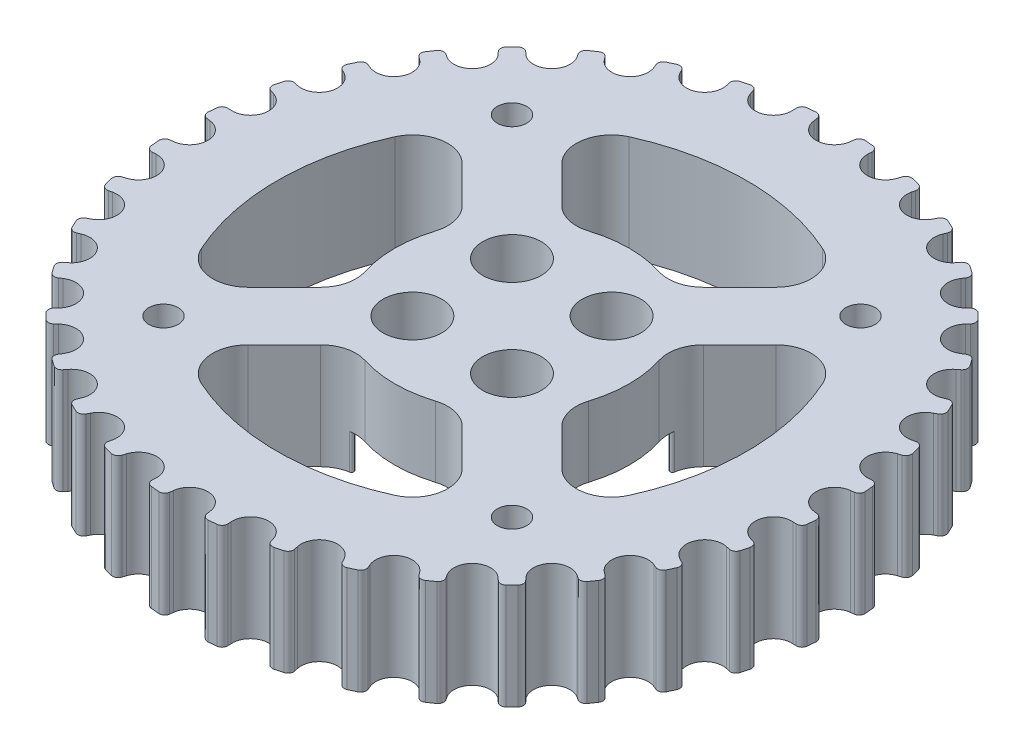
from build123d import *

# Parameters (mm, degrees)
CUT_EXTRUDE_1_DEPTH      = 46.197240435
PATTERN_CIRCULAR_1_COUNT = 36
CUT_EXTRUDE_START        = -2.5
SKETCH_3_R               = 41.846456916
CUT_EXTRUDE_2_DEPTH      = 2.5
SKETCH_4_R               = 25
EXTRUDE_1_DEPTH          = 9
CUT_EXTRUDE_START_2      = -6
SKETCH_5_R               = 29.365062609
CUT_EXTRUDE_3_DEPTH      = 6
SKETCH_6_R               = 2.5
SKETCH_6_R_2             = 1.25
CUT_EXTRUDE_4_DEPTH      = 10
SKETCH_8_R               = 10.05
CUT_EXTRUDE_6_DEPTH      = 3
FILLET_1_R               = 0.2


with BuildPart() as part:
    # 草图1 → 旋转1 (revolve)
    with BuildSketch(Plane.XY, mode=Mode.PRIVATE) as revolve_1_sk:
        Polygon((24, 0), (28.08, 0), (28.08, 9), (30.14789, 9), (30.14789, 11.5), (22.5, 11.5), (22.5, 4), (18, 4), (18, 3), (9, 3), (9, -2), (18.5, -2), (18.5, -6), (20, -6), (20, -5), (21, -5), (21, 2), (24, 2), align=None)
    revolve(revolve_1_sk.sketch.rotate(Axis((0, 0, 0), (0, 1, 0)), 90), axis=Axis((0, 0, 0), (0, 1, 0)))

    # 草图2 → 切除-拉伸1 (cut, through all)
    with BuildSketch(Plane.XZ.offset(-9)):
        with BuildLine():
            Line((-1.58417409, 27.581468475), (-1.548371997, 27.289883824))
            ThreePointArc((-1.548371997, 27.289883824), (0, 25.92), (1.548371997, 27.289883824))
            Line((1.548371997, 27.289883824), (1.58417409, 27.581468475))
            ThreePointArc((1.58417409, 27.581468475), (1.756189946, 27.894100287), (2.096432699, 28.001631559))
            ThreePointArc((2.096432699, 28.001631559), (0, 28.08), (-2.096432699, 28.001631559))
            ThreePointArc((-2.096432699, 28.001631559), (-1.756189946, 27.894100287), (-1.58417409, 27.581468475))
        make_face()
    cut_extrude_1 = extrude(amount=CUT_EXTRUDE_1_DEPTH, mode=Mode.SUBTRACT)

    # 阵列(圆周)1: 切除-拉伸1 ×36 about axis
    pattern_circular_1_axis = Axis((0, 0, 0), (0, 1, 0))
    for i in range(1, PATTERN_CIRCULAR_1_COUNT):
        add(cut_extrude_1.rotate(pattern_circular_1_axis, i * 360 / PATTERN_CIRCULAR_1_COUNT), mode=Mode.SUBTRACT)

    # 草图3 → 切除-拉伸2 (cut)
    with BuildSketch(Plane(origin=(0, 11.5, 0), x_dir=(1, 0, 0), z_dir=(0, 1, 0)).offset(CUT_EXTRUDE_START)):
        Circle(SKETCH_3_R)
    extrude(amount=CUT_EXTRUDE_2_DEPTH, mode=Mode.SUBTRACT)

    # 草图4 → 凸台-拉伸1 (add)
    with BuildSketch(Plane(origin=(0, 9, 0), x_dir=(1, 0, 0), z_dir=(0, 1, 0))):
        Circle(SKETCH_4_R)
    extrude(amount=-EXTRUDE_1_DEPTH)

    # 草图5 → 切除-拉伸3 (cut)
    with BuildSketch(Plane.XZ.offset(6).offset(CUT_EXTRUDE_START_2)):
        Circle(SKETCH_5_R)
    extrude(amount=CUT_EXTRUDE_3_DEPTH, mode=Mode.SUBTRACT)

    # 草图6 → 切除-拉伸4 (cut)
    with BuildSketch(Plane(origin=(0, 9, 0), x_dir=(1, 0, 0), z_dir=(0, 1, 0))):
        with Locations(Location((-4.242640687, 4.242640687, 0), (0, 0, 270))):
            Circle(SKETCH_6_R)
        with Locations(Location((4.242640687, 4.242640687, 0), (0, 0, 270))):
            Circle(SKETCH_6_R)
        with Locations(Location((-4.242640687, -4.242640687, 0), (0, 0, 270))):
            Circle(SKETCH_6_R)
        with Locations(Location((4.242640687, -4.242640687, 0), (0, 0, 270))):
            Circle(SKETCH_6_R)
        with Locations(Location((-14.849242405, 14.849242405, 0), (0, 0, 270))):
            Circle(SKETCH_6_R_2)
        with Locations(Location((14.849242405, 14.849242405, 0), (0, 0, 270))):
            Circle(SKETCH_6_R_2)
        with Locations(Location((14.849242405, -14.849242405, 0), (0, 0, 270))):
            Circle(SKETCH_6_R_2)
        with Locations(Location((-14.849242405, -14.849242405, 0), (0, 0, 270))):
            Circle(SKETCH_6_R_2)
        with BuildLine():
            Line((-6.033432872, 10.276073559), (-9.125901536, 13.368542223))
            ThreePointArc((-9.125901536, 13.368542223), (-9.955920686, 16.028003061), (-8.240683755, 18.223367725))
            ThreePointArc((-8.240683755, 18.223367725), (0, 20), (8.240683755, 18.223367725))
            ThreePointArc((8.240683755, 18.223367725), (9.955920686, 16.028003061), (9.125901536, 13.368542223))
            Line((9.125901536, 13.368542223), (6.033432872, 10.276073559))
            ThreePointArc((6.033432872, 10.276073559), (4.624825024, 9.483283249), (3.009317329, 9.536456848))
            ThreePointArc((3.009317329, 9.536456848), (0, 10), (-3.009317329, 9.536456848))
            ThreePointArc((-3.009317329, 9.536456848), (-4.624825024, 9.483283249), (-6.033432872, 10.276073559))
        make_face()
        with BuildLine():
            Line((-13.368542223, 9.125901536), (-10.276073559, 6.033432872))
            ThreePointArc((-10.276073559, 6.033432872), (-9.483283249, 4.624825024), (-9.536456848, 3.009317329))
            ThreePointArc((-9.536456848, 3.009317329), (-10, 0), (-9.536456848, -3.009317329))
            ThreePointArc((-9.536456848, -3.009317329), (-9.483283249, -4.624825024), (-10.276073559, -6.033432872))
            Line((-10.276073559, -6.033432872), (-13.368542223, -9.125901536))
            ThreePointArc((-13.368542223, -9.125901536), (-16.028003061, -9.955920686), (-18.223367725, -8.240683755))
            ThreePointArc((-18.223367725, -8.240683755), (-20, 0), (-18.223367725, 8.240683755))
            ThreePointArc((-18.223367725, 8.240683755), (-16.028003061, 9.955920686), (-13.368542223, 9.125901536))
        make_face()
        with BuildLine():
            Line((10.276073559, 6.033432872), (13.368542223, 9.125901536))
            ThreePointArc((13.368542223, 9.125901536), (16.028003061, 9.955920686), (18.223367725, 8.240683755))
            ThreePointArc((18.223367725, 8.240683755), (20, 0), (18.223367725, -8.240683755))
            ThreePointArc((18.223367725, -8.240683755), (16.028003061, -9.955920686), (13.368542223, -9.125901536))
            Line((13.368542223, -9.125901536), (10.276073559, -6.033432872))
            ThreePointArc((10.276073559, -6.033432872), (9.483283249, -4.624825024), (9.536456848, -3.009317329))
            ThreePointArc((9.536456848, -3.009317329), (10, 0), (9.536456848, 3.009317329))
            ThreePointArc((9.536456848, 3.009317329), (9.483283249, 4.624825024), (10.276073559, 6.033432872))
        make_face()
        with BuildLine():
            Line((6.033432872, -10.276073559), (9.125901536, -13.368542223))
            ThreePointArc((9.125901536, -13.368542223), (9.955920686, -16.028003061), (8.240683755, -18.223367725))
            ThreePointArc((8.240683755, -18.223367725), (0, -20), (-8.240683755, -18.223367725))
            ThreePointArc((-8.240683755, -18.223367725), (-9.955920686, -16.028003061), (-9.125901536, -13.368542223))
            Line((-9.125901536, -13.368542223), (-6.033432872, -10.276073559))
            ThreePointArc((-6.033432872, -10.276073559), (-4.624825024, -9.483283249), (-3.009317329, -9.536456848))
            ThreePointArc((-3.009317329, -9.536456848), (0, -10), (3.009317329, -9.536456848))
            ThreePointArc((3.009317329, -9.536456848), (4.624825024, -9.483283249), (6.033432872, -10.276073559))
        make_face()
    extrude(amount=-CUT_EXTRUDE_4_DEPTH, mode=Mode.SUBTRACT)

    # 草图8 → 切除-拉伸6 (cut)
    with BuildSketch(Plane.XZ):
        Circle(SKETCH_8_R)
    extrude(amount=-CUT_EXTRUDE_6_DEPTH, mode=Mode.SUBTRACT)

    # 圆角1
    fillet_1_edges = [part.edges().sort_by_distance(p)[0] for p in [
        (3.478133212, 1.5, 9.428949536),
        (9.428949536, 1.5, 3.478133212),
        (9.428949536, 1.5, -3.478133212),
        (3.478133212, 1.5, -9.428949536),
        (-9.428949536, 1.5, -3.478133212),
        (-3.478133212, 1.5, -9.428949536),
        (-9.428949536, 1.5, 3.478133212),
        (-3.478133212, 1.5, 9.428949536),
    ]]
    fillet(fillet_1_edges, radius=FILLET_1_R)


solid = part.part
